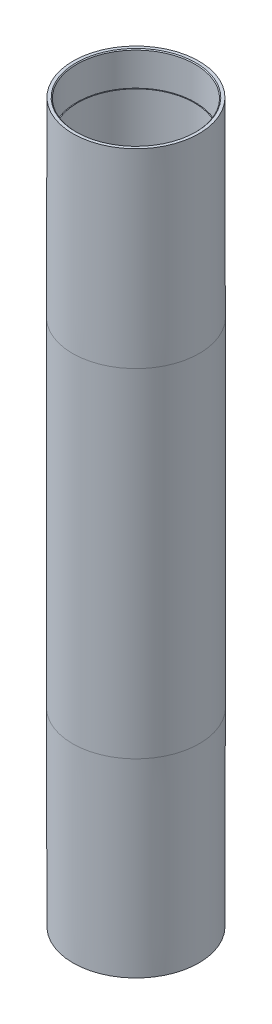
SolidWorks part; units mm, degrees
material "1023 碳钢板 (SS)"
ref_plane "前视基准面" through (0, 0, 0) normal (0, 0, 1) x (1, 0, 0)
ref_plane "上视基准面" through (0, 0, 0) normal (0, 1, 0) x (1, 0, 0)
ref_plane "右视基准面" through (0, 0, 0) normal (1, 0, 0) x (0, 0, -1)
sketch "草图1" plane through (0, 0, 0) normal (0, 0, 1) x (1, 0, 0)
  line L0 (0, 0) -> (-0.5, 225)
  line L1 (-0.5, 225) -> (-0.5, 625)
  line L2 (-0.5, 625) -> (0, 850)
  line L3 (0, 850) -> (74.5, 850)
  line L4 (0, 0) -> (74.5, 0)
  line L5 (74.5, 850) -> (74.5, 737.8515) construction
  line L6 (74.5, 0) -> (74.5, 850)
  dimension "D1" = 400
  dimension "D2" = 225
  dimension "D3" = 225
  dimension "D4" = 74.5
  dimension "D5" = 75
revolve "旋转1" add sketch "草图1" angle 360 about L5
sketch "草图2" plane through (0, 850, 0) normal (0, 1, 0) x (1, 0, 0)
  circle A0 centre (74.5, 0) radius 70
  dimension "D1" = 140
extrude "切除-拉伸1" cut sketch "草图2" against normal blind 40
sketch "草图3" plane through (0, 0, 0) normal (0, -1, 0) x (1, 0, 0)
  circle A0 centre (74.5, 0) radius 70
  dimension "D1" = 140
extrude "切除-拉伸2" cut sketch "草图3" against normal blind 40
sketch "草图4" plane through (0, 40, 0) normal (0, -1, 0) x (1, 0, 0)
  circle A0 centre (74.5, 0) radius 69
  dimension "D1" = 138
extrude "切除-拉伸3" cut sketch "草图4" against normal blind 843
chamfer "倒角1" distance 1 angle 45 2 edges at (74.5, 0, -70) (74.5, 850, 70)
